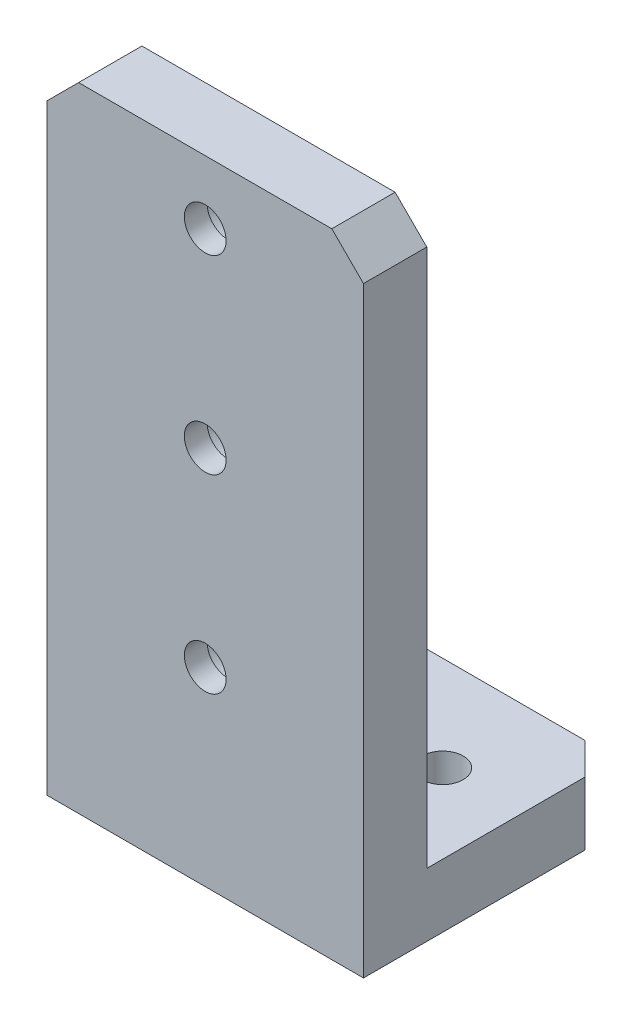
from build123d import *

# Parameters (mm, degrees)
EXTRUDE_2_DEPTH              = 25
HOLE_WIZARD_6_5_6_5_1_D      = 6.5
HOLE_WIZARD_M6_1_D           = 6.6
HOLE_WIZARD_M6_1_CBORE_D     = 11
HOLE_WIZARD_M6_1_CBORE_DEPTH = 6.4
CHAMFER_1_SIZE               = 5


with BuildPart() as part:
    # 草图2 → 拉伸-薄壁2 (new, symmetric)
    with BuildSketch(Plane(origin=(0, 0, 0), x_dir=(0, 0, -1), z_dir=(1, 0, 0))):
        Polygon((0, 100), (0, 0), (40, 0), (40, 10), (10, 10), (10, 100), align=None)
    extrude(amount=EXTRUDE_2_DEPTH, both=True)

    # Ø6.5 (6.5) 直径孔1 (through all)
    with Locations(Plane(origin=(0, 10, 0), x_dir=(1, 0, 0), z_dir=(0, 1, 0))):
        with Locations((-12.5, 25), (12.5, 25)):
            Hole(HOLE_WIZARD_6_5_6_5_1_D / 2)

    # M6 六角凹头螺钉的柱形沉头孔1 (through all)
    with Locations(Plane(origin=(0, 0, -10), x_dir=(-1, 0, 0), z_dir=(0, 0, -1))):
        with Locations((0, 90), (0, 60), (0, 30)):
            CounterBoreHole(HOLE_WIZARD_M6_1_D / 2, HOLE_WIZARD_M6_1_CBORE_D / 2, HOLE_WIZARD_M6_1_CBORE_DEPTH)

    # 倒角1
    chamfer_1_edges = [part.edges().sort_by_distance(p)[0] for p in [
        (25, 100, -5),
        (-25, 100, -5),
        (-25, 5, -40),
        (25, 5, -40),
    ]]
    chamfer(chamfer_1_edges, length=CHAMFER_1_SIZE)


solid = part.part
